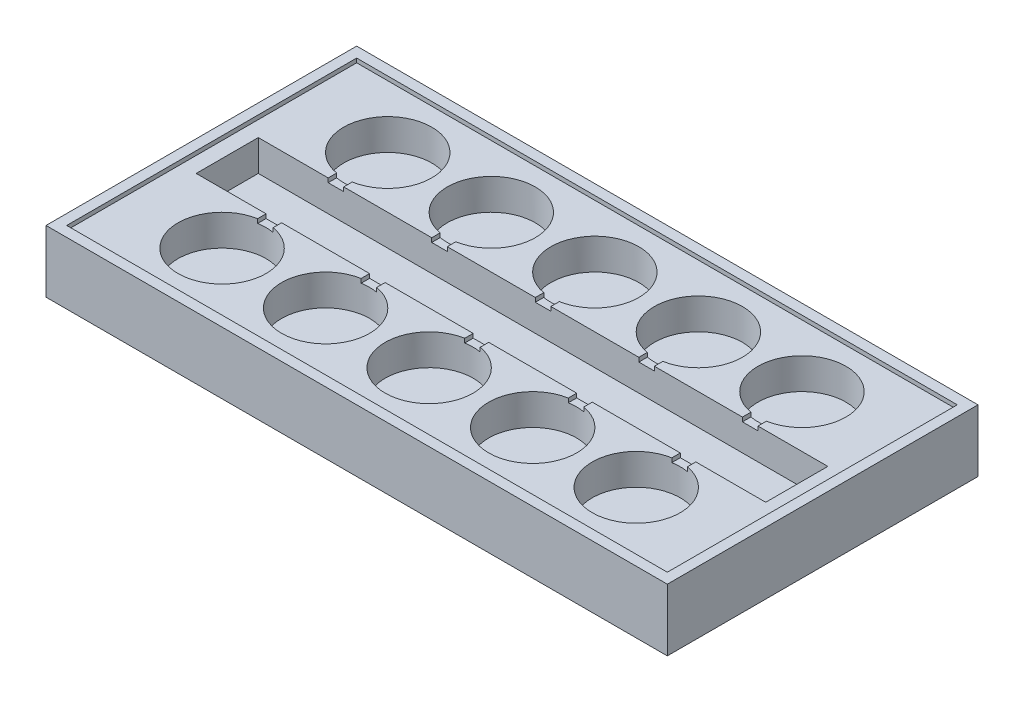
from build123d import *

# Parameters (mm, degrees)
SKETCH1_W           = 600
SKETCH1_H           = 300
BOSS_EXTRUDE1_DEPTH = 60
SKETCH2_R           = 42.5
SKETCH2_W           = 550
SKETCH2_H           = 60
CUT_EXTRUDE1_DEPTH  = 34
SKETCH3_W           = 580
SKETCH3_H           = 280
CUT_EXTRUDE2_DEPTH  = 4
SKETCH4_W           = 15
SKETCH4_H           = 96.703930486
CUT_EXTRUDE3_DEPTH  = 4
LPATTERN1_COUNT     = 3
LPATTERN1_PITCH     = 100
LPATTERN1_COL_COUNT = 3
LPATTERN1_COL_PITCH = 100


with BuildPart() as part:
    # Sketch1 → Boss-Extrude1 (new body)
    with BuildSketch(Plane(origin=(0, 0, 0), x_dir=(1, 0, 0), z_dir=(0, 1, 0))):
        Rectangle(SKETCH1_W, SKETCH1_H)
    extrude(amount=BOSS_EXTRUDE1_DEPTH)

    # Sketch2 → Cut-Extrude1 (cut)
    with BuildSketch(Plane(origin=(0, 60, 0), x_dir=(1, 0, 0), z_dir=(0, 1, 0))):
        with Locations(Location((0, 80, 0), (0, 0, 270))):
            Circle(SKETCH2_R)
        with Locations(Location((0, -80, 0), (0, 0, 90))):
            Circle(SKETCH2_R)
        with Locations(Location((-100, 80, 0), (0, 0, 270))):
            Circle(SKETCH2_R)
        with Locations(Location((-200, 80, 0), (0, 0, 270))):
            Circle(SKETCH2_R)
        with Locations(Location((200, 80, 0), (0, 0, 90))):
            Circle(SKETCH2_R)
        with Locations(Location((100, 80, 0), (0, 0, 90))):
            Circle(SKETCH2_R)
        with Locations(Location((200, -80, 0), (0, 0, 270))):
            Circle(SKETCH2_R)
        with Locations(Location((100, -80, 0), (0, 0, 270))):
            Circle(SKETCH2_R)
        with Locations(Location((-100, -80, 0), (0, 0, 90))):
            Circle(SKETCH2_R)
        with Locations(Location((-200, -80, 0), (0, 0, 90))):
            Circle(SKETCH2_R)
        Rectangle(SKETCH2_W, SKETCH2_H)
    extrude(amount=-CUT_EXTRUDE1_DEPTH, mode=Mode.SUBTRACT)

    # Sketch3 → Cut-Extrude2 (cut)
    with BuildSketch(Plane(origin=(0, 60, 0), x_dir=(1, 0, 0), z_dir=(0, 1, 0))):
        Rectangle(SKETCH3_W, SKETCH3_H)
    extrude(amount=-CUT_EXTRUDE2_DEPTH, mode=Mode.SUBTRACT)

    # Sketch4 → Cut-Extrude3 (cut)
    with BuildSketch(Plane(origin=(0, 56, 0), x_dir=(1, 0, 0), z_dir=(0, 1, 0))):
        Rectangle(SKETCH4_W, SKETCH4_H)
    cut_extrude3 = extrude(amount=-CUT_EXTRUDE3_DEPTH, mode=Mode.SUBTRACT)

    # LPattern1: Cut-Extrude3 ×3
    with Locations(*[(-i * LPATTERN1_PITCH, 0, 0) for i in range(1, LPATTERN1_COUNT)]):
        add(cut_extrude3, mode=Mode.SUBTRACT)

    # LPattern1 col: Cut-Extrude3 ×3
    with Locations(*[(i * LPATTERN1_COL_PITCH, 0, 0) for i in range(1, LPATTERN1_COL_COUNT)]):
        add(cut_extrude3, mode=Mode.SUBTRACT)


solid = part.part
